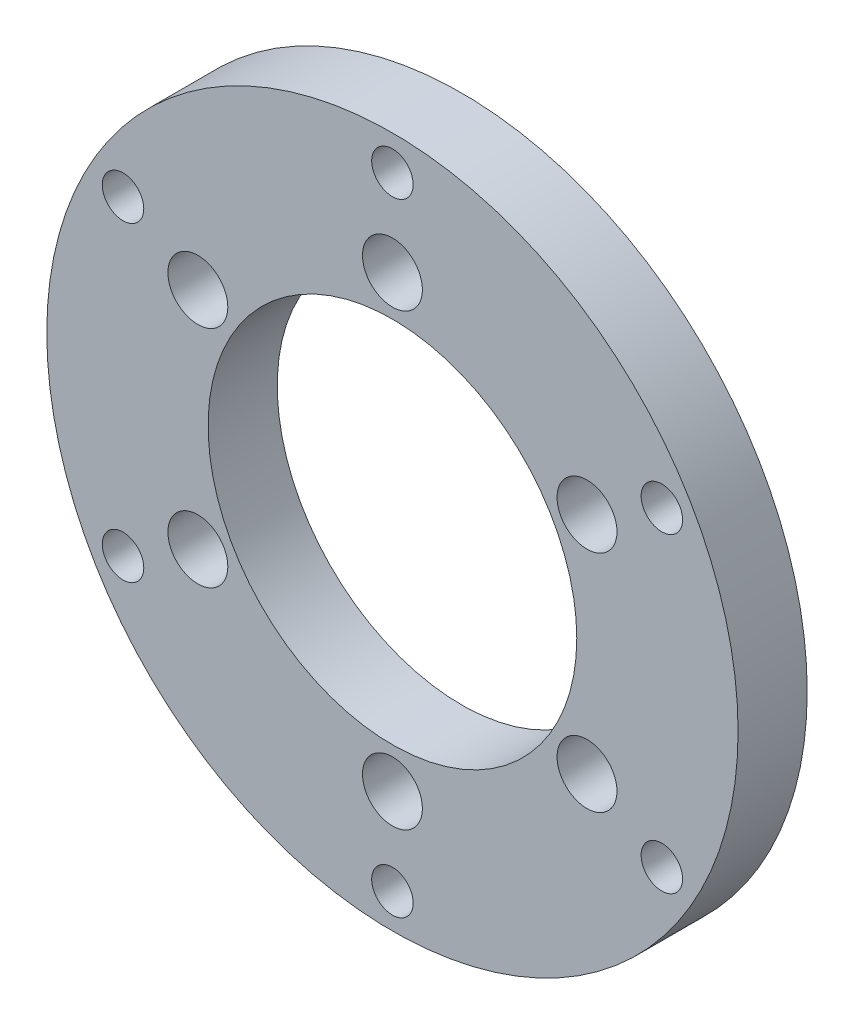
SolidWorks part; units mm, degrees
ref_plane "Front Plane" through (0, 0, 0) normal (0, 0, 1) x (1, 0, 0)
ref_plane "Top Plane" through (0, 0, 0) normal (0, 1, 0) x (1, 0, 0)
ref_plane "Right Plane" through (0, 0, 0) normal (1, 0, 0) x (0, 0, -1)
sketch "Sketch1" plane through (0, 0, 0) normal (0, 0, 1) x (1, 0, 0)
  circle A0 centre (0, 0) radius 150
  circle A1 centre (0, 0) radius 80
  dimension "D1" = 300
  dimension "D2" = 160
extrude "Boss-Extrude1" add sketch "Sketch1" along normal blind 30
sketch "Sketch2" plane through (0, 0, 30) normal (0, 0, 1) x (1, 0, 0)
  circle A0 centre (0, 0) radius 135 construction
  circle A1 centre (0, 135) radius 9
  circle A2 centre (116.9134, 67.5) radius 9
  circle A3 centre (116.9134, -67.5) radius 9
  circle A4 centre (0, -135) radius 9
  circle A5 centre (-116.9134, -67.5) radius 9
  circle A6 centre (-116.9134, 67.5) radius 9
  point P18 (0, 0)
  dimension "D1" = 270
  dimension "D2" = 18
extrude "Cut-Extrude1" cut sketch "Sketch2" against normal blind 30
sketch "Sketch3" plane through (0, 0, 30) normal (0, 0, 1) x (1, 0, 0)
  circle A0 centre (0, 0) radius 97.5 construction
  circle A1 centre (0, 97.5) radius 9
  circle A2 centre (84.4375, 48.75) radius 9
  circle A3 centre (84.4375, -48.75) radius 9
  circle A4 centre (0, -97.5) radius 9
  circle A5 centre (-84.4375, -48.75) radius 9
  circle A6 centre (-84.4375, 48.75) radius 9
  point P18 (0, 0)
  dimension "D1" = 195
  dimension "D2" = 18
extrude "Cut-Extrude2" cut sketch "Sketch3" against normal through all
sketch "Sketch4" plane through (0, 0, 30) normal (0, 0, 1) x (1, 0, 0)
  circle A0 centre (0, 97.5) radius 13
  circle A1 centre (84.4375, 48.75) radius 13
  circle A2 centre (84.4375, -48.75) radius 13
  circle A3 centre (0, -97.5) radius 13
  circle A4 centre (-84.4375, -48.75) radius 13
  circle A5 centre (-84.4375, 48.75) radius 13
  dimension "D1" = 26
extrude "Cut-Extrude3" cut sketch "Sketch4" against normal blind 20
